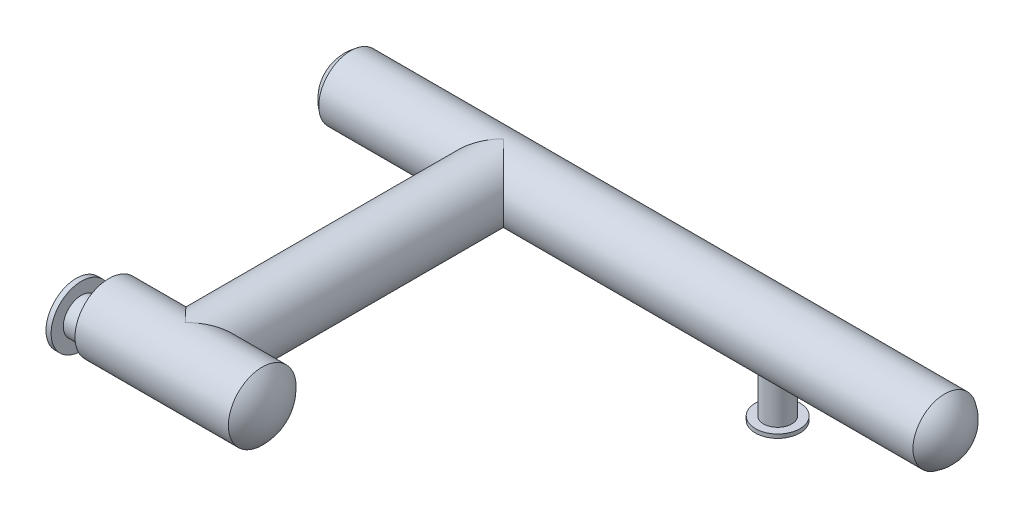
from build123d import *

# Parameters (mm, degrees)
SKETCH2_R           = 150
SKETCH2_R_2         = 140
BOSS_EXTRUDE1_DEPTH = 1500
SKETCH5_R           = 85
SKETCH5_R_2         = 79
BOSS_EXTRUDE2_DEPTH = 100
SKETCH6_R           = 142.5
SKETCH6_R_2         = 60.5
BOSS_EXTRUDE3_DEPTH = 24
SKETCH9_R           = 66.5
SKETCH9_R_2         = 60.5
BOSS_EXTRUDE4_DEPTH = 334
SKETCH10_R          = 105
SKETCH10_R_2        = 60.5
BOSS_EXTRUDE5_DEPTH = 18


with BuildPart() as part:
    # Sketch1 → Revolve1 (revolve)
    with BuildSketch(Plane.XY):
        with BuildLine():
            Line((159.844496112, 150), (2962.0029442, 150))
            ThreePointArc((2962.0029442, 150), (3024.61513919, 86.324033595), (3047.486013309, 0))
            Line((3047.486013309, 0), (3037.486013309, 0))
            ThreePointArc((3037.486013309, 0), (3016.591126725, 80.196062571), (2959.219584954, 140))
            Line((2959.219584954, 140), (162.906732213, 140))
            ThreePointArc((162.906732213, 140), (108.853694848, 79.07526069), (89.343239823, 0))
            Line((89.343239823, 0), (79.343239823, 0))
            ThreePointArc((79.343239823, 0), (100.740317612, 85.118229928), (159.844496112, 150))
        make_face()
    revolve(axis=Axis((0, 0, 0), (1, 0, 0)))

    # Sketch2 → Boss-Extrude1 (add)
    with BuildSketch(Plane.XY):
        with Locations((880, 0)):
            Circle(SKETCH2_R)
        with Locations((880, 0)):
            Circle(SKETCH2_R_2, mode=Mode.SUBTRACT)
    extrude(amount=BOSS_EXTRUDE1_DEPTH)

    # Sketch4 → Revolve2 (revolve)
    with BuildSketch(Plane.XY.offset(1500), mode=Mode.PRIVATE) as revolve2_sk:
        with BuildLine():
            Line((1243.197122588, 150), (519.922248056, 150))
            ThreePointArc((519.922248056, 150), (502.892003661, 70.895140734), (496.404784819, -9.761687714))
            Line((496.404784819, -9.761687714), (506.405833086, -9.761687714))
            ThreePointArc((506.405833086, -9.761687714), (512.258520744, 65.782083773), (527.516838947, 140))
            Line((527.516838947, 140), (1239.100117121, 140))
            ThreePointArc((1239.100117121, 140), (1284.368347054, 71.23548166), (1299.107077562, -9.761687714))
            Line((1299.107077562, -9.761687714), (1309.109201329, -9.761687714))
            ThreePointArc((1309.109201329, -9.761687714), (1292.821072695, 76.995752533), (1243.197122588, 150))
        make_face()
    revolve(revolve2_sk.sketch.rotate(Axis((496.404784819, -9.761687714, 1500), (1, 0, 0)), 180), axis=Axis((496.404784819, -9.761687714, 1500), (1, 0, 0)))



with BuildPart() as body_2:
    # Sketch5 → Boss-Extrude2 (new body)
    with BuildSketch(Plane(origin=(550, 0, 0), x_dir=(0, 0, -1), z_dir=(1, 0, 0))):
        with Locations((-1559.992129451, -8.789883245)):
            Circle(SKETCH5_R)
        with Locations((-1559.992129451, -8.789883245)):
            Circle(SKETCH5_R_2, mode=Mode.SUBTRACT)
    extrude(amount=-BOSS_EXTRUDE2_DEPTH)


with BuildPart() as part_1:
    add(part.part)

    add(body_2.part)  # Boss-Extrude3 merges body 2
    # Sketch6 → Boss-Extrude3 (add)
    with BuildSketch(Plane.ZY.offset(-450)):
        with Locations((1559.992129451, -8.789883245)):
            Circle(SKETCH6_R)
        with Locations((1559.992129451, -8.789883245)):
            Circle(SKETCH6_R_2, mode=Mode.SUBTRACT)
    extrude(amount=BOSS_EXTRUDE3_DEPTH)

    # Sketch9 → Boss-Extrude4 (add)
    with BuildSketch(Plane(origin=(0, 0, 0), x_dir=(1, 0, 0), z_dir=(0, 1, 0))):
        with Locations(Location((2174.0029442, 0, 0), (0, 0, 270))):
            Circle(SKETCH9_R)
        with Locations(Location((2174.0029442, 0, 0), (0, 0, 270))):
            Circle(SKETCH9_R_2, mode=Mode.SUBTRACT)
    extrude(amount=-BOSS_EXTRUDE4_DEPTH)

    # Sketch10 → Boss-Extrude5 (add)
    with BuildSketch(Plane(origin=(0, -334, 0), x_dir=(-1, 0, 0), z_dir=(0, -1, 0))):
        with Locations(Location((-2174.0029442, 0, 0), (0, 0, 90))):
            Circle(SKETCH10_R)
        with Locations(Location((-2174.0029442, 0, 0), (0, 0, 270))):
            Circle(SKETCH10_R_2, mode=Mode.SUBTRACT)
    extrude(amount=BOSS_EXTRUDE5_DEPTH)


solid = part_1.part
